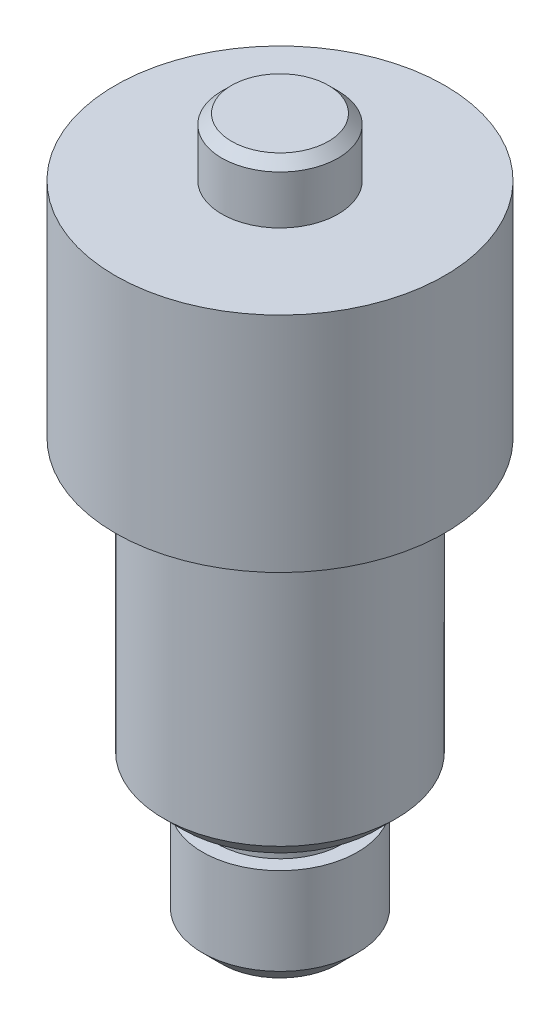
SolidWorks part; units mm, degrees
material "35"
ref_plane "前视基准面" through (0, 0, 0) normal (0, 0, 1) x (1, 0, 0)
ref_plane "上视基准面" through (0, 0, 0) normal (0, 1, 0) x (1, 0, 0)
ref_plane "右视基准面" through (0, 0, 0) normal (1, 0, 0) x (0, 0, -1)
sketch "草图1" plane through (0, 0, 0) normal (0, 0, 1) x (1, 0, 0)
  line L0 (0, 0) -> (6, 0)
  line L1 (6, 0) -> (6, -6)
  line L2 (6, -6) -> (17, -6)
  line L3 (17, -6) -> (17, -29)
  line L4 (17, -29) -> (12, -29)
  line L5 (12, -29) -> (12, -59)
  line L6 (12, -59) -> (6.5, -59)
  line L7 (6.5, -59) -> (6.5, -62)
  line L8 (6.5, -62) -> (8, -62)
  line L9 (8, -62) -> (8, -73)
  line L10 (8, -73) -> (0, -73)
  line L13 (0, -73) -> (0, 0)
  dimension "D1" = 6
  dimension "D2" = 6
  dimension "D3" = 23
  dimension "D4" = 3
  dimension "D5" = 73
  dimension "D7" = 17
  dimension "D8" = 12
  dimension "D9" = 6.5
  dimension "D11" = 8
  dimension "D12" = 30
revolve "旋转1" add sketch "草图1" angle 360 about L13
cosmetic thread "装饰螺纹线1" parameters "D2"=13.835
chamfer "倒角1" distance 2 angle 45 2 edges at (0, -59, -12) (0, -73, -8)
chamfer "倒角2" distance 1 angle 45 1 edges at (0, 0, -6)
fillet "圆角1" radius 0.3 1 edges at (0, -29, -12)
